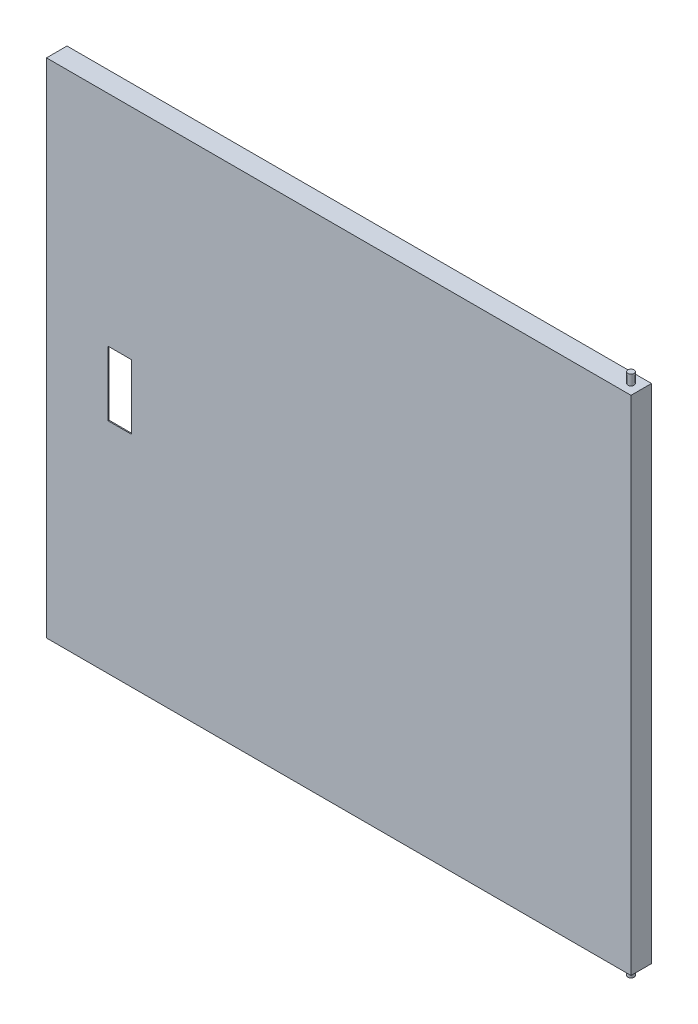
SolidWorks part; units mm, degrees
material "Q235"
ref_plane "前视基准面" through (0, 0, 0) normal (0, 0, 1) x (1, 0, 0)
ref_plane "上视基准面" through (0, 0, 0) normal (0, 1, 0) x (1, 0, 0)
ref_plane "右视基准面" through (0, 0, 0) normal (1, 0, 0) x (0, 0, -1)
sketch "草图1" plane through (0, 0, 0) normal (0, 0, 1) x (1, 0, 0)
  line L1 (-285, 245) -> (285, 245)
  line L2 (-285, 245) -> (-285, -245)
  line L3 (-285, -245) -> (285, -245)
  line L4 (285, 245) -> (285, -245)
  line L5 (-285, 245) -> (285, -245) construction
  line L6 (-285, -245) -> (285, 245) construction
  point P0 (0, 0)
  dimension "D1" = 570
  dimension "D2" = 490
extrude "凸台-拉伸1" add sketch "草图1" along normal blind 20
shell "抽壳3" thickness 1
sketch "草图5" plane through (0, 0, 0) normal (0, 0, -1) x (-1, 0, 0)
  line L0 (-275, 235) -> (-275, -235)
  line L1 (-285, 245) -> (285, 245)
  line L2 (-285, 245) -> (-285, -245)
  line L3 (-285, -245) -> (285, -245)
  line L4 (285, 245) -> (285, -245)
  line L5 (-275, -235) -> (275, -235)
  line L6 (275, 235) -> (275, -235)
  line L7 (-275, 235) -> (275, 235)
  dimension "D1" = 10
extrude "凸台-拉伸3" add sketch "草图5" against normal blind 1.5
sketch "草图11" plane through (0, 245, 0) normal (0, 1, 0) x (1, 0, 0)
  line L0 (285, -10) -> (271.3665, -10) construction
  line L1 (285, -20) -> (285, 0) construction
  circle A0 centre (275, -10) radius 3
  dimension "D1" = 6
  dimension "D2" = 10
extrude "凸台-拉伸4" add sketch "草图11" along normal blind 10
sketch "草图12" plane through (0, -245, 0) normal (0, -1, 0) x (1, 0, 0)
  circle A0 centre (275, 10) radius 3
  dimension "D1" = 6
extrude "凸台-拉伸5" add sketch "草图12" along normal blind 10
sketch "草图13" plane through (0, 0, 20) normal (0, 0, 1) x (1, 0, 0)
  line L0 (-285, 0) -> (285, 0) construction
  line L1 (-285, 245) -> (-285, -245) construction
  line L2 (285, -245) -> (285, 245) construction
  line L4 (-225, -31.5) -> (-202, -31.5)
  line L5 (-225, -31.5) -> (-225, 31.5)
  line L6 (-225, 31.5) -> (-202, 31.5)
  line L7 (-202, -31.5) -> (-202, 31.5)
  line L8 (-225, -31.5) -> (-202, 31.5) construction
  line L9 (-225, 31.5) -> (-202, -31.5) construction
  point P6 (-213.5, 0)
  dimension "D1" = 63
  dimension "D2" = 23
  dimension "D3" = 71.5
extrude "切除-拉伸3" cut sketch "草图13" against normal blind 1.5
